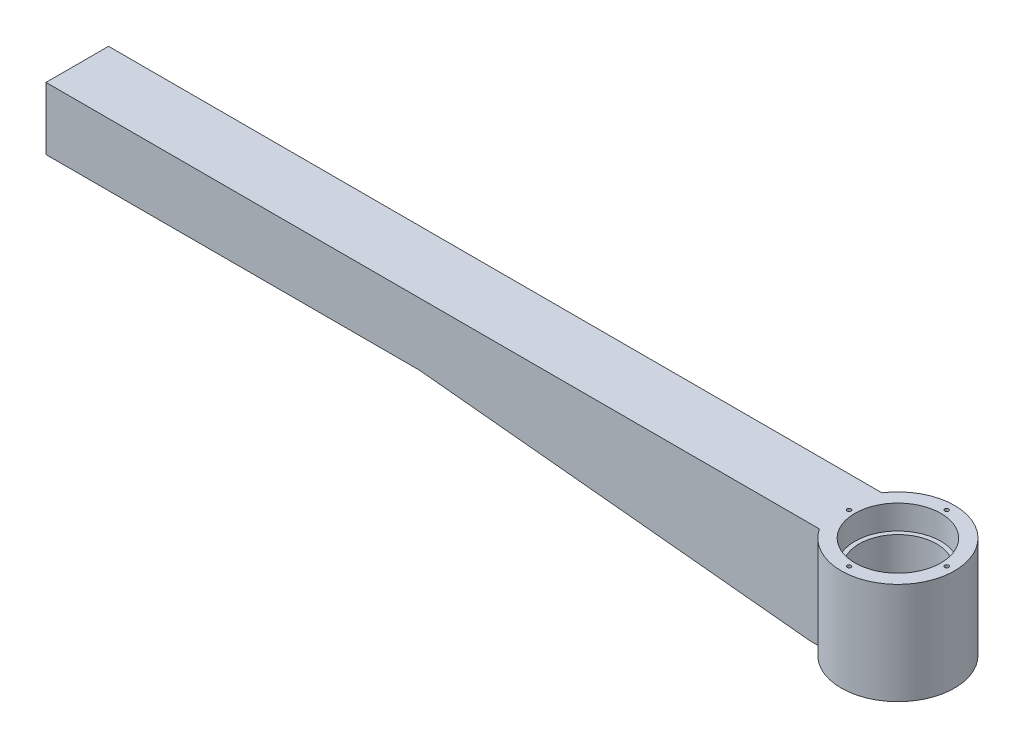
from build123d import *

# Parameters (mm, degrees)
CIRPATTERN1_COUNT   = 4
CIRPATTERN2_COUNT   = 4
BOSS_EXTRUDE1_DEPTH = 80
SHELL1_T            = -6
BOSS_EXTRUDE3_DEPTH = 6


with BuildPart() as part:
    # Sketch1 → Revolve1 (revolve)
    with BuildSketch(Plane.XY, mode=Mode.PRIVATE) as revolve1_sk:
        Polygon((-55, 0), (-72.5, 0), (-72.5, 130), (-55, 130), (-55, 99), (-49.5, 99), (-49.5, 31), (-55, 31), align=None)
    revolve(revolve1_sk.sketch.rotate(Axis((0, 0, 0), (0, 1, 0)), 270), axis=Axis((0, 0, 0), (0, 1, 0)))

    # Sketch2 → M6 Tapped Hole1 (revolve, cut)
    with BuildSketch(Plane(origin=(0, 130, -62.5), x_dir=(0, 0, 1), z_dir=(1, 0, 0))):
        Polygon((0, 0), (0, 19.502151548), (2.5, 18), (2.5, 0), align=None)
    m6_tapped_hole1 = revolve(axis=Axis((0, 136.35, -62.5), (0, -1, 0)), mode=Mode.SUBTRACT)

    # CirPattern1: M6 Tapped Hole1 ×4 about axis
    cirpattern1_axis = Axis((0, 0, 0), (0, 1, 0))
    for i in range(1, CIRPATTERN1_COUNT):
        add(m6_tapped_hole1.rotate(cirpattern1_axis, i * 360 / CIRPATTERN1_COUNT), mode=Mode.SUBTRACT)

    # Sketch4 → M6 Tapped Hole2 (revolve, cut)
    with BuildSketch(Plane(origin=(0, 0, 62.5), x_dir=(0, 0, -1), z_dir=(1, 0, 0))):
        Polygon((0, 0), (0, 19.502151548), (2.5, 18), (2.5, 0), align=None)
    m6_tapped_hole2 = revolve(axis=Axis((0, -6.35, 62.5), (0, 1, 0)), mode=Mode.SUBTRACT)

    # CirPattern2: M6 Tapped Hole2 ×4 about axis
    cirpattern2_axis = Axis((0, 0, 0), (0, 1, 0))
    for i in range(1, CIRPATTERN2_COUNT):
        add(m6_tapped_hole2.rotate(cirpattern2_axis, i * 360 / CIRPATTERN2_COUNT), mode=Mode.SUBTRACT)



with BuildPart() as body_2:
    # Sketch6 → Boss-Extrude1 (new body)
    with BuildSketch(Plane(origin=(0, 130, 0), x_dir=(1, 0, 0), z_dir=(0, 1, 0))):
        with BuildLine():
            Line((-1050, 40), (-60.466933112, 40))
            ThreePointArc((-60.466933112, 40), (-72.5, 0), (-60.466933112, -40))
            Line((-60.466933112, -40), (-1050, -40))
            Line((-1050, -40), (-1050, 40))
        make_face()
    extrude(amount=-BOSS_EXTRUDE1_DEPTH)

    # Shell1
    shell1_openings = [body_2.faces().sort_by_distance(p)[0] for p in [
        (-72.5, 90, 0),
        (-1050, 90, 0),
    ]]
    offset(amount=SHELL1_T, openings=shell1_openings, kind=Kind.INTERSECTION)


with BuildPart() as part_1:
    add(part.part)

    add(body_2.part)  # Boss-Extrude3 merges body 2
    # Sketch8 → Boss-Extrude3 (add)
    with BuildSketch(Plane.XY.offset(40)):
        Polygon((-60.466933112, 50), (-572.5, 50), (-72.5, 0), (-60.466933112, 0), align=None)
    boss_extrude3 = extrude(amount=-BOSS_EXTRUDE3_DEPTH)

    # Mirror1: Boss-Extrude3 across plane
    add(boss_extrude3.mirror(Plane.XY))


solid = part_1.part
